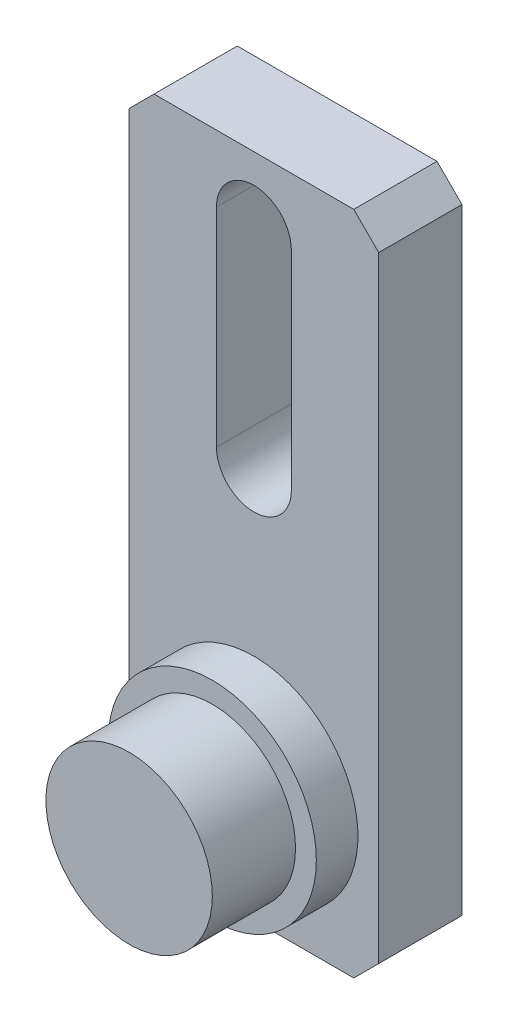
from build123d import *

# Parameters (mm, degrees)
SKETCH_1_W          = 30
SKETCH_1_H          = 80
EXTRUDE_1_DEPTH     = 10
SKETCH_2_R          = 12.5
EXTRUDE_2_DEPTH     = 15
CUT_EXTRUDE_START   = -10
SKETCH_3_R          = 12.5
SKETCH_3_R_2        = 10
CUT_EXTRUDE_1_DEPTH = 10
CUT_EXTRUDE_2_DEPTH = 46.276925691
CHAMFER_1_SIZE      = 3


with BuildPart() as part:
    # 草图1 → 凸台-拉伸1 (new body)
    with BuildSketch(Plane.XY):
        Rectangle(SKETCH_1_W, SKETCH_1_H)
    extrude(amount=EXTRUDE_1_DEPTH)

    # 草图2 → 凸台-拉伸2 (add)
    with BuildSketch(Plane.XY.offset(10)):
        with Locations(Location((0, -25, 0), (0, 0, 180))):
            Circle(SKETCH_2_R)
    extrude(amount=EXTRUDE_2_DEPTH)

    # 草图3 → 切除-拉伸1 (cut)
    with BuildSketch(Plane.XY.offset(25).offset(CUT_EXTRUDE_START)):
        with Locations(Location((0, -25, 0), (0, 0, 180))):
            Circle(SKETCH_3_R)
        with Locations((0, -25)):
            Circle(SKETCH_3_R_2, mode=Mode.SUBTRACT)
    extrude(amount=CUT_EXTRUDE_1_DEPTH, mode=Mode.SUBTRACT)

    # 草图4 → 切除-拉伸2 (cut, through all)
    with BuildSketch(Plane.XY.offset(10)):
        with BuildLine():
            Line((4.5, 32), (4.5, 7))
            ThreePointArc((4.5, 7), (0, 2.5), (-4.5, 7))
            Line((-4.5, 7), (-4.5, 32))
            ThreePointArc((-4.5, 32), (0, 36.5), (4.5, 32))
        make_face()
    extrude(amount=-CUT_EXTRUDE_2_DEPTH, mode=Mode.SUBTRACT)

    # 倒角1
    chamfer_1_edges = [part.edges().sort_by_distance(p)[0] for p in [
        (15, -40, 5),
        (-15, -40, 5),
        (-15, 40, 5),
        (15, 40, 5),
    ]]
    chamfer(chamfer_1_edges, length=CHAMFER_1_SIZE)


solid = part.part
